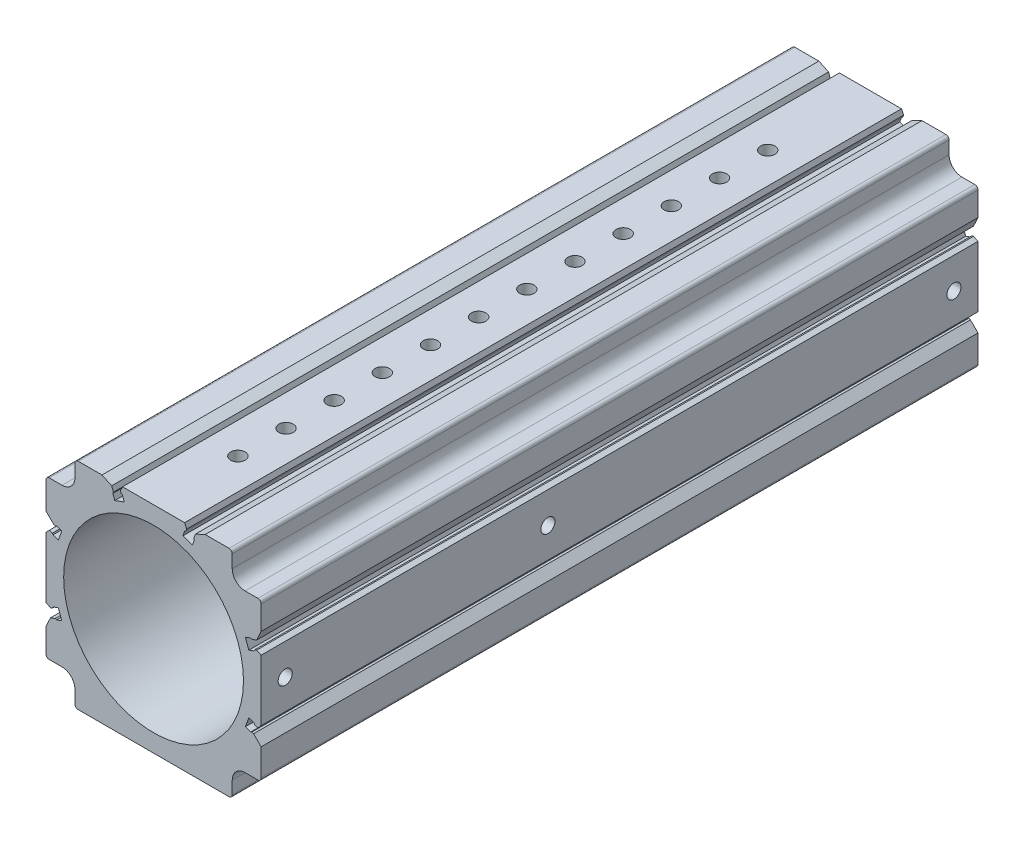
from build123d import *
from OCP.BRepFilletAPI import BRepFilletAPI_MakeChamfer

# Parameters (mm, degrees)
SKETCH1_R                 = 56
BOSS_EXTRUDE1_DEPTH       = 446.5
SKETCH3_W                 = 24.000744141
SKETCH3_H                 = 31.311653019
CUT_EXTRUDE2_DEPTH        = 457.443041353
FILLET1_R                 = 8
CIRPATTERN1_COUNT         = 4
FILLET1_OF_CIRPATTERN1_R  = 8
LPATTERN1_COUNT           = 12
LPATTERN1_PITCH           = 30
G1_8_TAPPED_HOLE1_D       = 8.8
G1_8_TAPPED_HOLE1_DEPTH   = 22.18
G1_8_TAPPED_HOLE1_TIP     = 2.643786724
FILLET2_R                 = 2
G1_8_TAPPED_HOLE2_D       = 8.8
G1_8_TAPPED_HOLE2_DEPTH   = 22.18
G1_8_TAPPED_HOLE2_TIP     = 2.643786724
CUT_EXTRUDE4_DEPTH        = 457.443041481
BOSS_EXTRUDE3_DEPTH       = 446.5
CHAMFER2_SIZE             = 3
CHAMFER2_SIZE2            = 2.340618026
CHAMFER3_SIZE             = 3
CHAMFER3_SIZE2            = 5.019471555
CHAMFER2_OF_MIRROR1_SIZE2 = 2.340618026
CHAMFER2_OF_MIRROR1_SIZE  = 3
CHAMFER3_OF_MIRROR1_SIZE2 = 5.019471555
CHAMFER3_OF_MIRROR1_SIZE  = 3
CIRPATTERN13_COUNT        = 4
CIRPATTERN14_COUNT        = 4
MIRROR2_COPY_1_DEPTH      = 457.443041481
MIRROR2_COPY_2_DEPTH      = 457.443041481
BOSS_EXTRUDE4_DEPTH       = 446.5
CHAMFER4_SIZE             = 3
CHAMFER4_SIZE2            = 2.340618026
CHAMFER4_SIZE2_2          = 5.019471555


with BuildPart() as part:
    # Sketch1 → Boss-Extrude1 (new body)
    with BuildSketch(Plane.XY):
        with BuildLine():
            Line((-44.8, 67), (-36.913248654, 67))
            Line((-36.913248654, 67), (-32.6, 67))
            Line((-32.6, 67), (-32.6, 66.1))
            Line((-32.6, 66.1), (-33.2, 65.5))
            Line((-33.2, 65.5), (-33.2, 62))
            Line((-33.2, 62), (-26.9, 62))
            Line((-26.9, 62), (-26.9, 65.5))
            Line((-26.9, 65.5), (-27.5, 66.1))
            Line((-27.5, 66.1), (-27.5, 67))
            Line((-27.5, 67), (27.5, 67))
            Line((27.5, 67), (27.5, 66.1))
            Line((27.5, 66.1), (26.9, 65.5))
            Line((26.9, 65.5), (26.9, 62))
            Line((26.9, 62), (33.2, 62))
            Line((33.2, 62), (33.2, 65.5))
            Line((33.2, 65.5), (32.6, 66.1))
            Line((32.6, 66.1), (32.6, 67))
            Line((32.6, 67), (36.913248654, 67))
            Line((36.913248654, 67), (44.8, 67))
            Line((44.8, 67), (57, 67))
            ThreePointArc((57, 67), (64.071067812, 64.071067812), (67, 57))
            Line((67, 57), (67, 44.8))
            Line((67, 44.8), (67, 36.913248654))
            Line((67, 36.913248654), (67, 32.6))
            Line((67, 32.6), (66.1, 32.6))
            Line((66.1, 32.6), (65.5, 33.2))
            Line((65.5, 33.2), (62, 33.2))
            Line((62, 33.2), (62, 26.9))
            Line((62, 26.9), (65.5, 26.9))
            Line((65.5, 26.9), (66.1, 27.5))
            Line((66.1, 27.5), (67, 27.5))
            Line((67, 27.5), (67, -27.5))
            Line((67, -27.5), (66.1, -27.5))
            Line((66.1, -27.5), (65.5, -26.9))
            Line((65.5, -26.9), (62, -26.9))
            Line((62, -26.9), (62, -33.2))
            Line((62, -33.2), (65.5, -33.2))
            Line((65.5, -33.2), (66.1, -32.6))
            Line((66.1, -32.6), (67, -32.6))
            Line((67, -32.6), (67, -36.913248654))
            Line((67, -36.913248654), (67, -44.8))
            Line((67, -44.8), (67, -57))
            ThreePointArc((67, -57), (64.071067812, -64.071067812), (57, -67))
            Line((57, -67), (44.8, -67))
            Line((44.8, -67), (36.913248654, -67))
            Line((36.913248654, -67), (-36.913248654, -67))
            Line((-36.913248654, -67), (-44.8, -67))
            Line((-44.8, -67), (-57, -67))
            ThreePointArc((-57, -67), (-64.071067812, -64.071067812), (-67, -57))
            Line((-67, -57), (-67, -44.8))
            Line((-67, -44.8), (-67, -36.913248654))
            Line((-67, -36.913248654), (-67, -32.6))
            Line((-67, -32.6), (-66.1, -32.6))
            Line((-66.1, -32.6), (-65.5, -33.2))
            Line((-65.5, -33.2), (-62, -33.2))
            Line((-62, -33.2), (-62, -26.9))
            Line((-62, -26.9), (-65.5, -26.9))
            Line((-65.5, -26.9), (-66.1, -27.5))
            Line((-66.1, -27.5), (-67, -27.5))
            Line((-67, -27.5), (-67, 27.5))
            Line((-67, 27.5), (-66.1, 27.5))
            Line((-66.1, 27.5), (-65.5, 26.9))
            Line((-65.5, 26.9), (-62, 26.9))
            Line((-62, 26.9), (-62, 33.2))
            Line((-62, 33.2), (-65.5, 33.2))
            Line((-65.5, 33.2), (-66.1, 32.6))
            Line((-66.1, 32.6), (-67, 32.6))
            Line((-67, 32.6), (-67, 36.913248654))
            Line((-67, 36.913248654), (-67, 44.8))
            Line((-67, 44.8), (-67, 57))
            ThreePointArc((-67, 57), (-64.071067812, 64.071067812), (-57, 67))
            Line((-57, 67), (-44.8, 67))
        make_face()
        Circle(SKETCH1_R, mode=Mode.SUBTRACT)
    extrude(amount=BOSS_EXTRUDE1_DEPTH)

    # Sketch3 → Cut-Extrude2 (cut, through all)
    with BuildSketch(Plane.XY.offset(446.5)):
        with Locations((-61.00037207, 64.65582651)):
            Rectangle(SKETCH3_W, SKETCH3_H)
    cut_extrude2 = extrude(amount=-CUT_EXTRUDE2_DEPTH, mode=Mode.SUBTRACT)

    # Fillet1
    fillet1_edges = [part.edges().sort_by_distance(p)[0] for p in [
        (-49, 49, 223.25),
    ]]
    fillet(fillet1_edges, radius=FILLET1_R)

    # CirPattern1: Cut-Extrude2 ×4 about axis
    cirpattern1_axis = Axis((0, 0, 0), (0, 0, 1))
    for i in range(1, CIRPATTERN1_COUNT):
        add(cut_extrude2.rotate(cirpattern1_axis, i * 360 / CIRPATTERN1_COUNT), mode=Mode.SUBTRACT)

    # Fillet1 of CirPattern1
    fillet1_of_cirpattern1_edges = [part.edges().sort_by_distance(p)[0] for p in [
        (-49, -49, 223.25),
        (49, -49, 223.25),
        (49, 49, 223.25),
    ]]
    fillet(fillet1_of_cirpattern1_edges, radius=FILLET1_OF_CIRPATTERN1_R)

    # Sketch8 → Ø9.0 (9) Diameter Hole1 (revolve, cut)
    with BuildSketch(Plane(origin=(0, 67, 394), x_dir=(0, 0, 1), z_dir=(1, 0, 0))):
        Polygon((0, 0), (0, 22.703872786), (4.5, 20), (4.5, 0), align=None)
    f_9_0_9_diameter_hole1 = revolve(axis=Axis((0, 73.35, 394), (0, -1, 0)), mode=Mode.SUBTRACT)

    # LPattern1: Ø9.0 (9) Diameter Hole1 ×12
    with Locations(*[(0, 0, -i * LPATTERN1_PITCH) for i in range(1, LPATTERN1_COUNT)]):
        add(f_9_0_9_diameter_hole1, mode=Mode.SUBTRACT)

    # G1/8 Tapped Hole1
    with Locations(Plane(origin=(67, 0, 0), x_dir=(0, 0, -1), z_dir=(1, 0, 0))):
        with Locations((-267.9, 0)):
            Hole(G1_8_TAPPED_HOLE1_D / 2, depth=G1_8_TAPPED_HOLE1_DEPTH)
            with Locations((0, 0, -(G1_8_TAPPED_HOLE1_DEPTH + G1_8_TAPPED_HOLE1_TIP / 2))):  # 118° drill point
                Cone(0, G1_8_TAPPED_HOLE1_D / 2, G1_8_TAPPED_HOLE1_TIP, mode=Mode.SUBTRACT)

    # Fillet2
    fillet2_edges = [part.edges().sort_by_distance(p)[0] for p in [
        (-67, 49, 223.25),
        (-49, 67, 223.25),
        (49, 67, 223.25),
        (67, 49, 223.25),
        (67, -49, 223.25),
        (-49, -67, 223.25),
        (49, -67, 223.25),
        (-67, -49, 223.25),
    ]]
    fillet(fillet2_edges, radius=FILLET2_R)

    # G1/8 Tapped Hole2
    with Locations(Plane(origin=(67, 0, 0), x_dir=(0, 0, -1), z_dir=(1, 0, 0))):
        with Locations((-431.5, 0), (-15, 0)):
            Hole(G1_8_TAPPED_HOLE2_D / 2, depth=G1_8_TAPPED_HOLE2_DEPTH)
            with Locations((0, 0, -(G1_8_TAPPED_HOLE2_DEPTH + G1_8_TAPPED_HOLE2_TIP / 2))):  # 118° drill point
                Cone(0, G1_8_TAPPED_HOLE2_D / 2, G1_8_TAPPED_HOLE2_TIP, mode=Mode.SUBTRACT)

    # Sketch25 → Cut-Extrude4 (cut, through all)
    with BuildSketch(Plane.XY.offset(446.5)):
        Polygon((-18.245217131, 59.33830594), (-24.165280642, 57.183579037), (-25.362351143, 60.47250321), (-25.003747657, 61.241530868), (-27.490726906, 68.074450198), (-22.69829454, 69.818752929), (-20.211315291, 62.985833599), (-19.442287632, 62.627230113), align=None)
    cut_extrude4 = extrude(amount=-CUT_EXTRUDE4_DEPTH, mode=Mode.SUBTRACT)

    # Sketch26 → Boss-Extrude3 (add, through all)
    with BuildSketch(Plane.XY.offset(446.5)):
        Polygon((-27.5, 67), (-26.290037253, 64.429630239), (-26.460290585, 61.340748366), (-34.000080984, 61.14617313), (-34.000080984, 67), align=None)
    boss_extrude3 = extrude(amount=-BOSS_EXTRUDE3_DEPTH)

    # Chamfer2
    chamfer2_edges = [part.edges().sort_by_distance(p)[0] for p in [
        (-21.672352376, 67, 223.25),
    ]]
    chamfer2_side = [part.faces().sort_by_distance(p)[0] for p in [
        (-20.941833833, 64.9929168, 223.25),
    ]]
    chamfer(chamfer2_edges, length=CHAMFER2_SIZE, length2=CHAMFER2_SIZE2, reference=chamfer2_side[0])

    # Chamfer3
    chamfer3_edges = [part.edges().sort_by_distance(p)[0] for p in [
        (-27.099659016, 67, 223.25),
    ]]
    chamfer3_side = [part.faces().sort_by_distance(p)[0] for p in [
        (-26.051703336, 64.120765434, 223.25),
    ]]
    chamfer(chamfer3_edges, length=CHAMFER3_SIZE, length2=CHAMFER3_SIZE2, reference=chamfer3_side[0])

    # Mirror1: Cut-Extrude4, Boss-Extrude3 across plane
    add(cut_extrude4.mirror(Plane(origin=(0, 0, 0), x_dir=(0, 0, 1), z_dir=(1, 0, 0))), mode=Mode.SUBTRACT)
    add(boss_extrude3.mirror(Plane(origin=(0, 0, 0), x_dir=(0, 0, 1), z_dir=(1, 0, 0))))

    # Chamfer2 of Mirror1
    chamfer2_of_mirror1_edges = [part.edges().sort_by_distance(p)[0] for p in [
        (21.672352376, 67, 223.25),
    ]]
    chamfer(chamfer2_of_mirror1_edges, length=CHAMFER2_OF_MIRROR1_SIZE, length2=CHAMFER2_OF_MIRROR1_SIZE2)

    # Chamfer3 of Mirror1
    chamfer3_of_mirror1_edges = [part.edges().sort_by_distance(p)[0] for p in [
        (27.099659016, 67, 223.25),
    ]]
    chamfer(chamfer3_of_mirror1_edges, length=CHAMFER3_OF_MIRROR1_SIZE, length2=CHAMFER3_OF_MIRROR1_SIZE2)

    # CirPattern13: Cut-Extrude4 ×4 about axis, 1 skipped
    cirpattern13_axis = Axis((0, 0, 0), (0, 0, 1))
    add([cut_extrude4.rotate(cirpattern13_axis, i * 360 / CIRPATTERN13_COUNT) for i in range(1, CIRPATTERN13_COUNT) if i not in (2,)], mode=Mode.SUBTRACT)

    # CirPattern14: Boss-Extrude3 ×4 about axis, 1 skipped
    cirpattern14_axis = Axis((0, 0, 446.5), (0, 0, -1))
    add([boss_extrude3.rotate(cirpattern14_axis, i * 360 / CIRPATTERN14_COUNT) for i in range(1, CIRPATTERN14_COUNT) if i not in (2,)])

    # Mirror2: Cut-Extrude4 across plane
    add(cut_extrude4.mirror(Plane.ZX), mode=Mode.SUBTRACT)

    # Mirror2 copy 1 sketch → Mirror2 copy 1 (cut, through all)
    with BuildSketch(Plane(origin=(0, 0, 446.5), x_dir=(0, -1, 0), z_dir=(0, 0, 1))):
        Polygon((-18.245217131, -59.33830594), (-24.165280642, -57.183579037), (-25.362351143, -60.47250321), (-25.003747657, -61.241530868), (-27.490726906, -68.074450198), (-22.69829454, -69.818752929), (-20.211315291, -62.985833599), (-19.442287632, -62.627230113), align=None)
    extrude(amount=-MIRROR2_COPY_1_DEPTH, mode=Mode.SUBTRACT)

    # Mirror2 copy 2 sketch → Mirror2 copy 2 (cut, through all)
    with BuildSketch(Plane(origin=(0, 0, 446.5), x_dir=(0, 1, 0), z_dir=(0, 0, 1))):
        Polygon((-18.245217131, -59.33830594), (-24.165280642, -57.183579037), (-25.362351143, -60.47250321), (-25.003747657, -61.241530868), (-27.490726906, -68.074450198), (-22.69829454, -69.818752929), (-20.211315291, -62.985833599), (-19.442287632, -62.627230113), align=None)
    extrude(amount=-MIRROR2_COPY_2_DEPTH, mode=Mode.SUBTRACT)

    # Sketch28 → Boss-Extrude4 (add, through all)
    with BuildSketch(Plane.XY.offset(446.5)):
        Polygon((-27.099659016, -67), (-21.672352376, -67), (-15.195943719, -57.916615682), (-28.958307841, -52.946873083), align=None)
        Polygon((-67, 27.5), (-67, 32.6), (-62.005583505, 35.167109027), (-60.064602607, 33.164833995), (-60.766437336, 26.614322888), (-64.028289916, 26.614322888), (-65.677432045, 26.791015241), align=None)
        Polygon((67, -27.5), (67, -32.6), (64.418272864, -34.192896025), (60.864105342, -33.812095479), (60.640482132, -29.234927503), (60.919197603, -26.633561815), (64.751432098, -26.446333253), (66.168921553, -27.078779421), align=None)
    extrude(amount=-BOSS_EXTRUDE4_DEPTH)

    # Chamfer4: one chamfer whose edges measure the first distance from different faces: ONE call of the kernel's chamfer builder (chamfer() names one face for all edges)
    chamfer4_edges_1 = [part.edges().sort_by_distance(p)[0] for p in [
        (-67, -21.672352376, 223.25),
    ]]
    chamfer4_side_1 = [part.faces().sort_by_distance(p)[0] for p in [
        (-64.9929168, -20.941833833, 223.25),
    ]]
    chamfer4_edges_2 = [part.edges().sort_by_distance(p)[0] for p in [
        (-67, -27.099659016, 223.25),
    ]]
    chamfer4_side_2 = [part.faces().sort_by_distance(p)[0] for p in [
        (-64.120765434, -26.051703336, 223.25),
    ]]
    chamfer4_edges_3 = [part.edges().sort_by_distance(p)[0] for p in [
        (67, 21.672352376, 223.25),
    ]]
    chamfer4_side_3 = [part.faces().sort_by_distance(p)[0] for p in [
        (64.9929168, 20.941833833, 223.25),
    ]]
    chamfer4_edges_4 = [part.edges().sort_by_distance(p)[0] for p in [
        (67, 27.099659016, 223.25),
    ]]
    chamfer4_side_4 = [part.faces().sort_by_distance(p)[0] for p in [
        (64.120765434, 26.051703336, 223.25),
    ]]
    chamfer4_edges_5 = [part.edges().sort_by_distance(p)[0] for p in [
        (-67, 27.099659016, 223.25),
    ]]
    chamfer4_side_5 = [part.faces().sort_by_distance(p)[0] for p in [
        (-67, 37.049829508, 223.25),
    ]]
    chamfer4_edges_6 = [part.edges().sort_by_distance(p)[0] for p in [
        (-67, 21.672352376, 223.25),
    ]]
    chamfer4_side_6 = [part.faces().sort_by_distance(p)[0] for p in [
        (-67, 0, 223.25),
    ]]
    chamfer4_edges_7 = [part.edges().sort_by_distance(p)[0] for p in [
        (67, -27.099659016, 223.25),
    ]]
    chamfer4_side_7 = [part.faces().sort_by_distance(p)[0] for p in [
        (67, -37.049829508, 223.25),
    ]]
    chamfer4_edges_8 = [part.edges().sort_by_distance(p)[0] for p in [
        (67, -21.672352376, 223.25),
    ]]
    chamfer4_side_8 = [part.faces().sort_by_distance(p)[0] for p in [
        (67, 0, 223.108344604),
    ]]
    chamfer4 = BRepFilletAPI_MakeChamfer(part.part.solid().wrapped)
    for e in chamfer4_edges_1:
        chamfer4.Add(CHAMFER4_SIZE, CHAMFER4_SIZE2, e.wrapped, chamfer4_side_1[0].wrapped)  # the first distance lies on this face
    for e in chamfer4_edges_2:
        chamfer4.Add(CHAMFER4_SIZE, CHAMFER4_SIZE2_2, e.wrapped, chamfer4_side_2[0].wrapped)  # the first distance lies on this face
    for e in chamfer4_edges_3:
        chamfer4.Add(CHAMFER4_SIZE, CHAMFER4_SIZE2, e.wrapped, chamfer4_side_3[0].wrapped)  # the first distance lies on this face
    for e in chamfer4_edges_4:
        chamfer4.Add(CHAMFER4_SIZE, CHAMFER4_SIZE2_2, e.wrapped, chamfer4_side_4[0].wrapped)  # the first distance lies on this face
    for e in chamfer4_edges_5:
        chamfer4.Add(CHAMFER4_SIZE, CHAMFER4_SIZE2_2, e.wrapped, chamfer4_side_5[0].wrapped)  # the first distance lies on this face
    for e in chamfer4_edges_6:
        chamfer4.Add(CHAMFER4_SIZE, CHAMFER4_SIZE2, e.wrapped, chamfer4_side_6[0].wrapped)  # the first distance lies on this face
    for e in chamfer4_edges_7:
        chamfer4.Add(CHAMFER4_SIZE, CHAMFER4_SIZE2_2, e.wrapped, chamfer4_side_7[0].wrapped)  # the first distance lies on this face
    for e in chamfer4_edges_8:
        chamfer4.Add(CHAMFER4_SIZE, CHAMFER4_SIZE2, e.wrapped, chamfer4_side_8[0].wrapped)  # the first distance lies on this face
    add(Compound.cast(chamfer4.Shape()), mode=Mode.REPLACE)


solid = part.part
